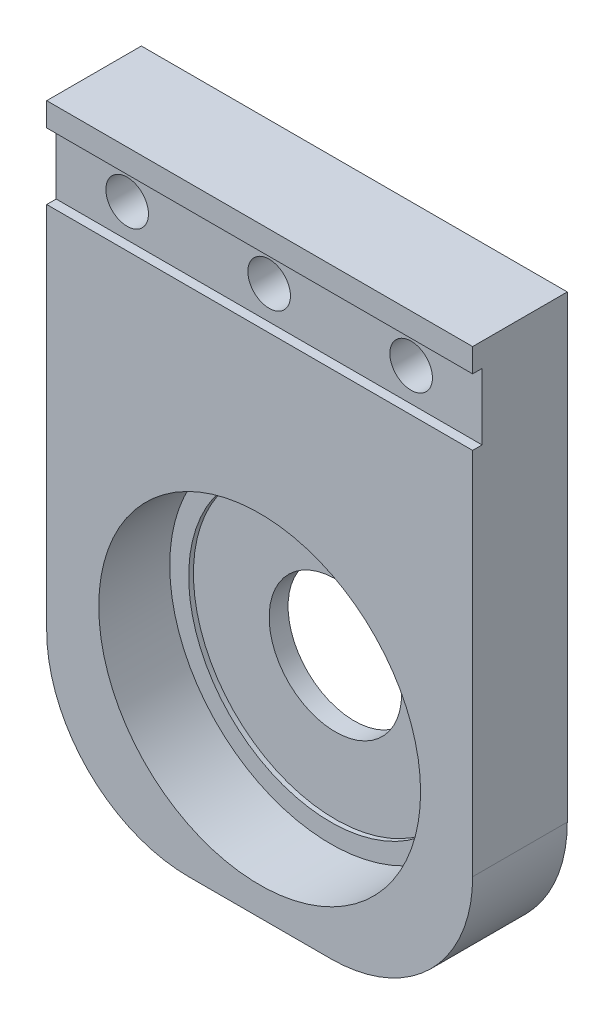
SolidWorks part; units mm, degrees
ref_plane "Front Plane" through (0, 0, 0) normal (0, 0, 1) x (1, 0, 0)
ref_plane "Top Plane" through (0, 0, 0) normal (0, 1, 0) x (1, 0, 0)
ref_plane "Right Plane" through (0, 0, 0) normal (1, 0, 0) x (0, 0, -1)
other "Configuration Table"
sketch "Sketch1" plane through (0, 0, 0) normal (0, 0, 1) x (1, 0, 0)
  line L1 (-45, 60) -> (45, 60)
  line L2 (-45, 60) -> (-45, -60)
  line L3 (-45, -60) -> (45, -60)
  line L4 (45, 60) -> (45, -60)
  line L5 (-45, 60) -> (45, -60) construction
  line L6 (-45, -60) -> (45, 60) construction
  point P0 (0, 0)
  dimension "D1" = 90
  dimension "D2" = 120
extrude "Boss-Extrude1" add sketch "Sketch1" along normal blind 20
sketch "Sketch2" plane through (0, 0, 20) normal (0, 0, 1) x (1, 0, 0)
  circle A0 centre (0, -20) radius 34
  dimension "D1" = 68
  dimension "D2" = 20
extrude "Cut-Extrude1" cut sketch "Sketch2" against normal blind 15
sketch "Sketch3" plane through (0, 0, 5) normal (0, 0, 1) x (1, 0, 0)
  circle A0 centre (0, -20) radius 30
  dimension "D1" = 60
extrude "Cut-Extrude2" cut sketch "Sketch3" against normal blind 1
sketch "Sketch4" plane through (0, 0, 4) normal (0, 0, 1) x (1, 0, 0)
  circle A0 centre (0, -20) radius 14
  dimension "D1" = 28
extrude "Cut-Extrude3" cut sketch "Sketch4" against normal blind 10
other "Move Face1" face at (0, 60, 10) parameters "D1"=2.02
fillet "Fillet1" radius 30 2 edges at (45, -60, 10) (-45, -60, 10)
other "Move Face2" face at (0, 62.02, 10) parameters "D1"=5
sketch "Sketch5" plane through (0, 0, 0) normal (0, 0, -1) x (-1, 0, 0)
  line L0 (-45, 55.02) -> (45, 55.02)
  line L1 (-45, -30) -> (-45, 67.02) construction
  line L2 (45, 67.02) -> (45, -30) construction
  line L3 (-45, 67.02) -> (45, 67.02) construction
  point P8 (-30, 55.02)
  point P9 (0, 55.02)
  point P10 (30, 55.02)
  dimension "D1" = 12
  dimension "D2" = 15
  dimension "D3" = 15
hole_wizard "CBORE for M8 Hexagon socket head cap screws1" positions "Sketch5" profile "Sketch6" counterbore size "M8" standard "GB"
sketch "Sketch6" plane through (-30, 55.02, 0) normal (1, 0, 0) x (0, 1, 0)
  line L0 (0, 0) -> (0, 82.9539)
  line L1 (0, 82.9539) -> (4.5, 80.25)
  line L2 (4.5, 80.25) -> (4.5, 9)
  line L3 (4.5, 9) -> (7.5, 9)
  line L4 (7.5, 9) -> (7.5, 0)
  line L5 (7.5, 0) -> (0, 0)
  line L10 (0, 82.9539) -> (-4.5, 80.25) construction
  line L11 (0, -6.35) -> (0, 107.95) construction
  dimension "孔直径" = 9
  dimension "孔深度" = 80.25
  dimension "柱形沉头孔直径" = 15
  dimension "柱形沉头孔深度" = 9
  dimension "导头角度" = 118
sketch "Sketch7" plane through (0, 0, 20) normal (0, 0, 1) x (1, 0, 0)
  line L0 (-45, 67.02) -> (-45, -30) construction
  line L1 (-45, 62.02) -> (45, 62.02)
  line L2 (-45, 62.02) -> (-45, 48.02)
  line L3 (-45, 48.02) -> (45, 48.02)
  line L4 (45, 62.02) -> (45, 48.02)
  line L5 (45, -30) -> (45, 67.02) construction
  line L6 (45, 67.02) -> (-45, 67.02) construction
  dimension "D1" = 5
  dimension "D2" = 14
extrude "Cut-Extrude4" cut sketch "Sketch7" against normal blind 2
